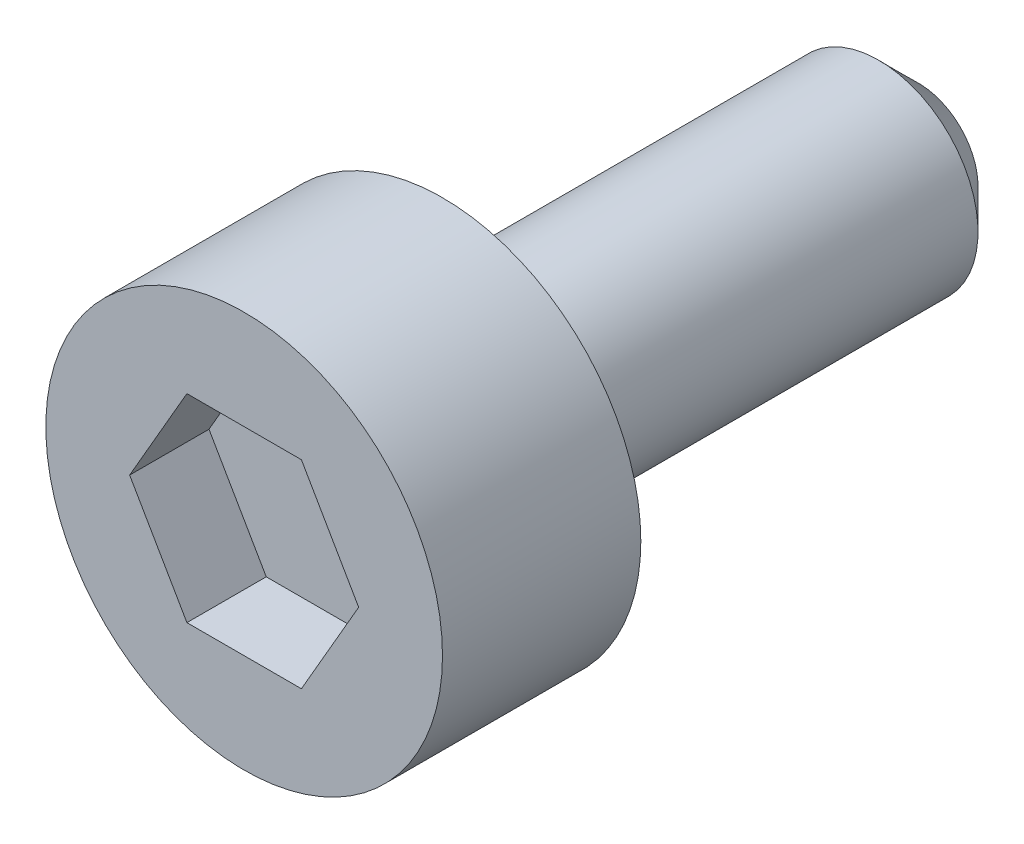
from build123d import *

# Parameters (mm, degrees)
SKETCH1_R           = 5
BOSS_EXTRUDE1_DEPTH = 5
CUT_EXTRUDE1_DEPTH  = 2
SKETCH3_R           = 2.5
BOSS_EXTRUDE2_DEPTH = 12
CHAMFER1_SIZE       = 1


with BuildPart() as part:
    # Sketch1 → Boss-Extrude1 (new body)
    with BuildSketch(Plane.XY):
        Circle(SKETCH1_R)
    extrude(amount=BOSS_EXTRUDE1_DEPTH)

    # Sketch2 → Cut-Extrude1 (cut)
    with BuildSketch(Plane.XY.offset(5)):
        Polygon((2.886751346, 0), (1.443375673, 2.5), (-1.443375673, 2.5), (-2.886751346, 0), (-1.443375673, -2.5), (1.443375673, -2.5), align=None)
    extrude(amount=-CUT_EXTRUDE1_DEPTH, mode=Mode.SUBTRACT)

    # Sketch3 → Boss-Extrude2 (add)
    with BuildSketch(Plane(origin=(0, 0, 0), x_dir=(-1, 0, 0), z_dir=(0, 0, -1))):
        Circle(SKETCH3_R)
    extrude(amount=BOSS_EXTRUDE2_DEPTH)

    # Chamfer1
    chamfer1_edges = [part.edges().sort_by_distance(p)[0] for p in [
        (2.5, 0, -12),
    ]]
    chamfer(chamfer1_edges, length=CHAMFER1_SIZE)


solid = part.part
